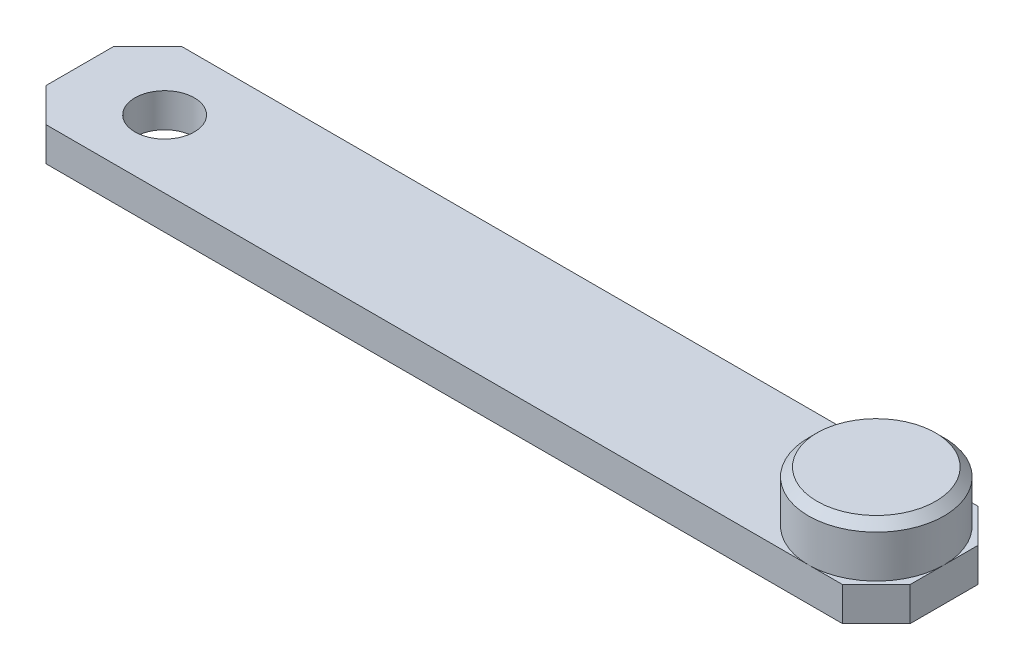
SolidWorks part; units mm, degrees
ref_plane "Front Plane" through (0, 0, 0) normal (0, 0, 1) x (1, 0, 0)
ref_plane "Top Plane" through (0, 0, 0) normal (0, 1, 0) x (1, 0, 0)
ref_plane "Right Plane" through (0, 0, 0) normal (1, 0, 0) x (0, 0, -1)
sketch "Sketch1" plane through (0, 0, 0) normal (0, 1, 0) x (1, 0, 0)
  line L1 (0, 8) -> (51, 8)
  line L2 (0, 8) -> (0, 0)
  line L3 (0, 0) -> (51, 0)
  line L4 (51, 8) -> (51, 0)
  dimension "D1" = 51
  dimension "D2" = 8
extrude "Boss-Extrude1" add sketch "Sketch1" along normal blind 2
sketch "Sketch2" plane through (0, 2, 0) normal (0, 1, 0) x (1, 0, 0)
  line L0 (51, 8) -> (0, 8) construction
  line L1 (0, 8) -> (0, 0) construction
  circle A0 centre (5, 4) radius 1.75
  dimension "D3" = 3.5
  dimension "D1" = 4
  dimension "D2" = 5
extrude "Cut-Extrude1" cut sketch "Sketch2" against normal through all
sketch "Sketch3" plane through (0, 2, 0) normal (0, 1, 0) x (1, 0, 0)
  line L0 (51, 8) -> (0, 8) construction
  line L1 (51, 0) -> (51, 8) construction
  circle A0 centre (47, 4) radius 4
  dimension "D2" = 4
  dimension "D3" = 8
  dimension "D1" = 4
extrude "Boss-Extrude2" add sketch "Sketch3" along normal blind 3
chamfer "Chamfer1" distance 0.5 angle 45 1 edges at (47, 5, 0)
chamfer "Chamfer2" distance 2 angle 45 4 edges at (51, 1, -8) (51, 1, 0) (0, 1, -8) (0, 1, 0)
